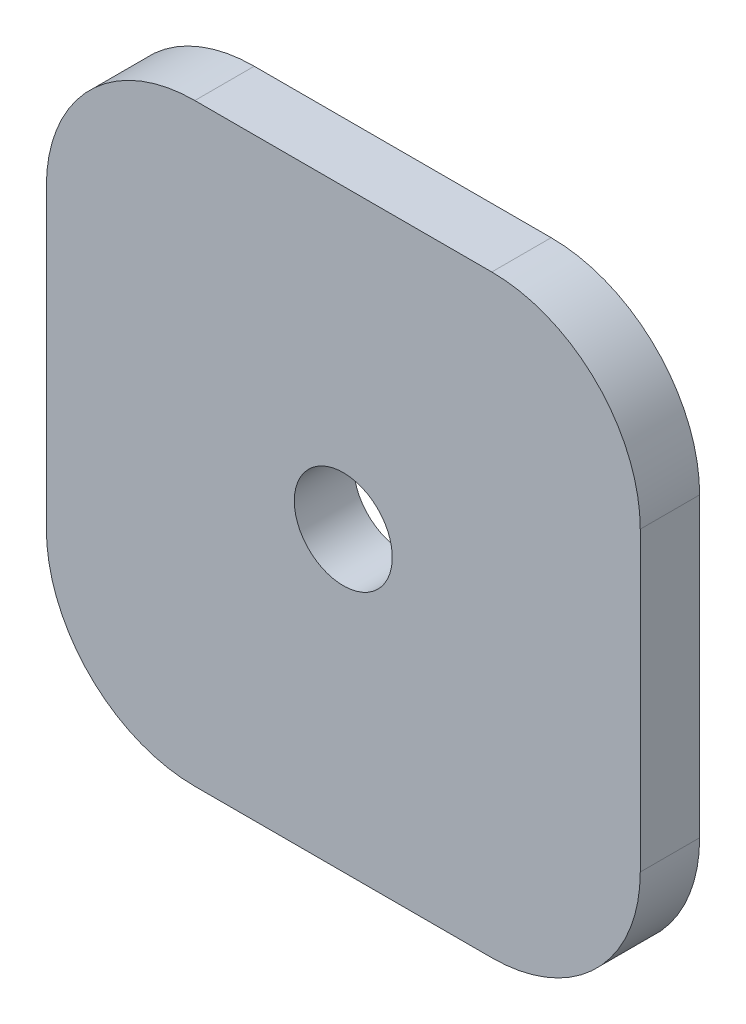
SolidWorks part; units mm, degrees
material "6061 GB/T6892-2006"
ref_plane "前视基准面" through (0, 0, 0) normal (0, 0, 1) x (1, 0, 0)
ref_plane "上视基准面" through (0, 0, 0) normal (0, 1, 0) x (1, 0, 0)
ref_plane "右视基准面" through (0, 0, 0) normal (1, 0, 0) x (0, 0, -1)
sketch "草图1" plane through (0, 0, 0) normal (0, 0, 1) x (1, 0, 0)
  line L5 (-20, 20) -> (20, 20)
  line L6 (-20, 20) -> (-20, -20)
  line L7 (-20, -20) -> (20, -20)
  line L8 (20, 20) -> (20, -20)
  line L9 (-20, 20) -> (20, -20) construction
  line L10 (-20, -20) -> (20, 20) construction
  point P0 (0, 0)
  dimension "D1" = 40
  dimension "D2" = 40
extrude "凸台-拉伸1" add sketch "草图1" along normal blind 4
fillet "圆角1" radius 10 4 edges at (20, 20, 2) (20, -20, 2) (-20, 20, 2) (-20, -20, 2)
hole_wizard "M6 螺纹孔1" positions "草图3" profile "草图4" tap size "M6" standard "GB"
sketch "草图3" plane through (0, 0, 4) normal (0, 0, 1) x (1, 0, 0)
  line L0 (-80, 22) -> (-80, -22) construction
  line L3 (0, 0) -> (48.6927, 0) construction
  point P0 (-60, 25)
  point P2 (-60, -25)
  point P4 (47, 25)
  point P6 (47, -25)
  dimension "D1" = 20
  dimension "D2" = 50
  dimension "D3" = 20
  dimension "D4" = 107
sketch "草图4" plane through (-60, 25, 4) normal (1, 0, 0) x (0, -1, 0)
  line L0 (0, 0) -> (0, 4)
  line L1 (0, 4) -> (2.5, 4)
  line L2 (2.5, 4) -> (2.5, 0)
  line L5 (2.5, 0) -> (0, 0)
  line L11 (0, -6.35) -> (0, 107.95) construction
  dimension "通孔螺纹孔钻头直径" = 5
  dimension "通孔螺纹孔钻头深度" = 4
cosmetic thread "孔螺蚊线1" [suppressed] parameters "D2"=6
cosmetic thread "孔螺蚊线2" [suppressed] parameters "D2"=6
cosmetic thread "孔螺蚊线3" [suppressed] parameters "D2"=6
cosmetic thread "孔螺蚊线4" [suppressed] parameters "D2"=6
hole_wizard "打孔尺寸(%根据)内六角花形半沉头螺钉的类型2" positions "草图5" profile "草图6" countersink size "M6" standard "GB"
sketch "草图5" plane through (0, 0, 0) normal (0, 0, -1) x (-1, 0, 0)
  line L0 (80, 10) -> (80, -10) construction
  point P0 (-52, 0)
  point P2 (8, 0)
  dimension "D1" = 72
  dimension "D2" = 60
sketch "草图6" plane through (52, 0, 0) normal (1, 0, 0) x (0, 1, 0)
  line L0 (0, 0) -> (0, 4)
  line L1 (0, 4) -> (3.3, 4)
  line L2 (3.3, 4) -> (3.3, 3.1)
  line L3 (3.3, 3.1) -> (6.4, 0)
  line L5 (6.4, 0) -> (0, 0)
  line L6 (-3.3, 3.1) -> (-6.4, 0) construction
  line L11 (0, -6.35) -> (0, 107.95) construction
  dimension "通孔孔直径" = 6.6
  dimension "通孔孔深度" = 4
  dimension "近端锥形沉头孔直径" = 12.8
  dimension "近端锥形沉头孔角度" = 90
hole_wizard "M6 间隙孔1" positions "草图7" profile "草图8" hole size "M6" standard "GB" end condition through all
sketch "草图7" plane through (0, 0, 0) normal (0, 0, -1) x (-1, 0, 0)
  point P0 (0, 0)
sketch "草图8" plane through (0, 0, 0) normal (1, 0, 0) x (0, 1, 0)
  line L0 (0, 0) -> (0, 4)
  line L1 (0, 4) -> (3.3, 4)
  line L2 (3.3, 4) -> (3.3, 0)
  line L5 (3.3, 0) -> (0, 0)
  line L11 (0, -6.35) -> (0, 107.95) construction
  dimension "通孔孔直径" = 6.6
  dimension "通孔孔深度" = 4
